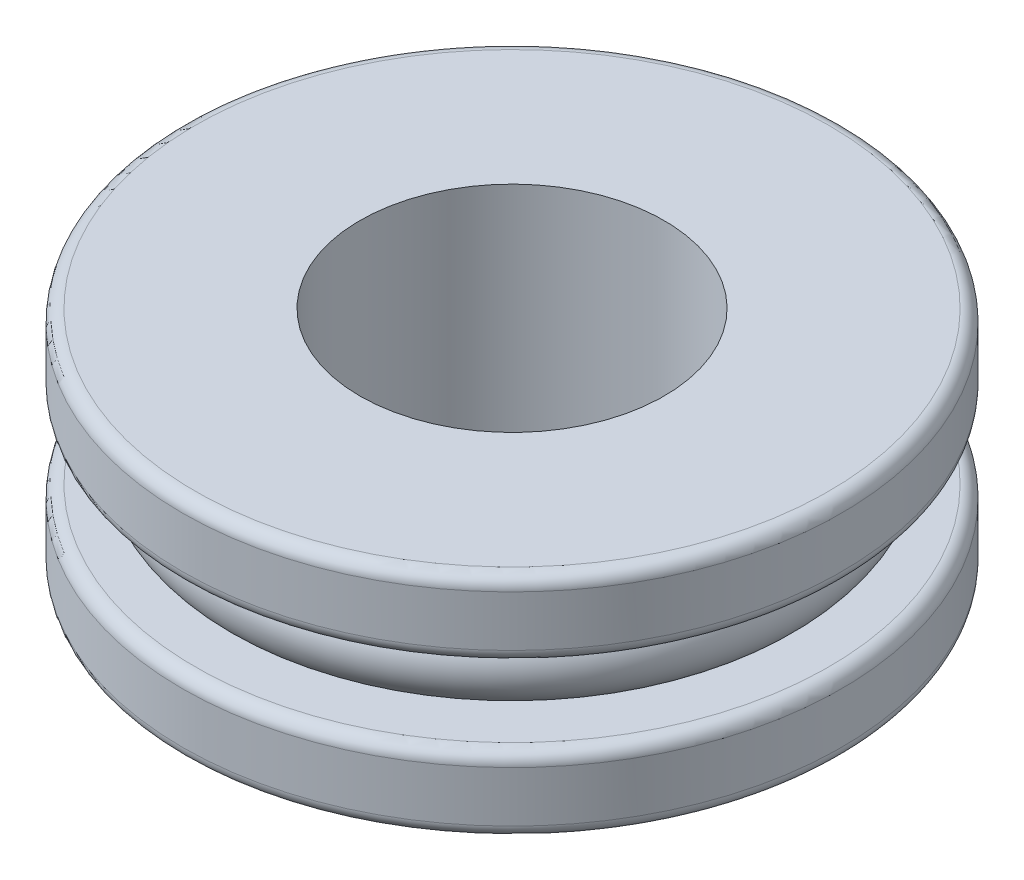
from build123d import *

# Parameters (mm, degrees)
FILLET1_R = 0.5


with BuildPart() as part:
    # Sketch1 → Revolve1 (revolve)
    with BuildSketch(Plane.XY, mode=Mode.PRIVATE) as revolve1_sk:
        with BuildLine():
            Line((6, 0), (13, 0))
            Line((13, 0), (13, -3))
            Line((13, -3), (10, -3))
            ThreePointArc((10, -3), (11.5, -4.5), (10, -6))
            Line((10, -6), (13, -6))
            Line((13, -6), (13, -9))
            Line((13, -9), (6, -9))
            Line((6, -9), (6, 0))
        make_face()
    revolve(revolve1_sk.sketch.rotate(Axis((0, 0, 0), (0, -1, 0)), 90), axis=Axis((0, 0, 0), (0, -1, 0)))

    # Fillet1
    fillet1_edges = [part.edges().sort_by_distance(p)[0] for p in [
        (0, 0, -13),
        (0, -9, -13),
        (0, -6, -13),
        (0, -3, -13),
    ]]
    fillet(fillet1_edges, radius=FILLET1_R)


solid = part.part
